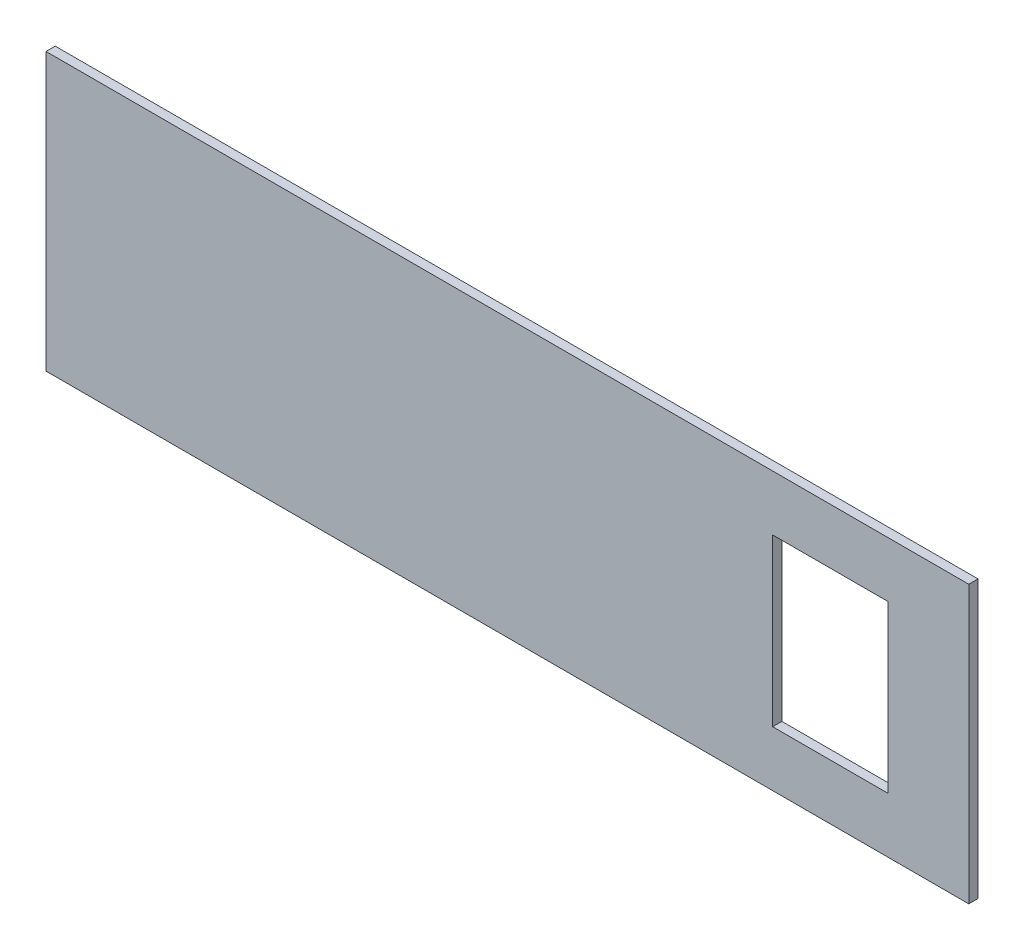
from build123d import *

# Parameters (mm, degrees)
SKETCH1_W              = 2000
SKETCH1_H              = 600
BOSS_EXTRUDE1_DEPTH    = 20
SKETCH2_W              = 250
SKETCH2_H              = 360
CUT_EXTRUDE1_DEPTH     = 1045.222198577
SKETCH3_W              = 60
SKETCH3_H              = 50
BOSS_EXTRUDE2_DEPTH    = 51
SKETCH4_W              = 60
SKETCH4_H              = 12
CUT_EXTRUDE2_DEPTH     = 40
FILLET1_R              = 12
SKETCH5_R              = 10
CUT_EXTRUDE3_DEPTH     = 1060.885489098
LPATTERN1_COUNT        = 2
LPATTERN1_PITCH        = 120
FILLET1_OF_LPATTERN1_R = 12


with BuildPart() as part:
    # Sketch1 → Boss-Extrude1 (new body)
    with BuildSketch(Plane.XY):
        Rectangle(SKETCH1_W, SKETCH1_H)
    extrude(amount=BOSS_EXTRUDE1_DEPTH)

    # Sketch2 → Cut-Extrude1 (cut, through all)
    with BuildSketch(Plane(origin=(0, 0, 0), x_dir=(-1, 0, 0), z_dir=(0, 0, -1))):
        with Locations((-700, 0)):
            Rectangle(SKETCH2_W, SKETCH2_H)
    extrude(amount=-CUT_EXTRUDE1_DEPTH, mode=Mode.SUBTRACT)

    # Sketch3 → Boss-Extrude2 (add)
    with BuildSketch(Plane(origin=(0, 0, 0), x_dir=(-1, 0, 0), z_dir=(0, 0, -1))):
        with Locations((-350, -22.5)):
            Rectangle(SKETCH3_W, SKETCH3_H)
    boss_extrude2 = extrude(amount=BOSS_EXTRUDE2_DEPTH)

    # Sketch4 → Cut-Extrude2 (cut)
    with BuildSketch(Plane(origin=(0, 0, -51), x_dir=(-1, 0, 0), z_dir=(0, 0, -1))):
        with Locations((-350, -23.5)):
            Rectangle(SKETCH4_W, SKETCH4_H)
    cut_extrude2 = extrude(amount=-CUT_EXTRUDE2_DEPTH, mode=Mode.SUBTRACT)

    # Fillet1
    fillet1_edges = [part.edges().sort_by_distance(p)[0] for p in [
        (380, -7.5, -51),
        (320, -38.5, -51),
        (380, -38.5, -51),
        (320, -7.5, -51),
    ]]
    fillet(fillet1_edges, radius=FILLET1_R)

    # Sketch5 → Cut-Extrude3 (cut, through all)
    with BuildSketch(Plane.XZ.offset(47.5)):
        with Locations((350, -26)):
            Circle(SKETCH5_R)
    cut_extrude3 = extrude(amount=-CUT_EXTRUDE3_DEPTH, mode=Mode.SUBTRACT)

    # LPattern1: Boss-Extrude2, Cut-Extrude2, Cut-Extrude3 ×2
    with Locations(*[(-i * LPATTERN1_PITCH, 0, 0) for i in range(1, LPATTERN1_COUNT)]):
        add(boss_extrude2)
        add(cut_extrude2, mode=Mode.SUBTRACT)
        add(cut_extrude3, mode=Mode.SUBTRACT)

    # Fillet1 of LPattern1
    fillet1_of_lpattern1_edges = [part.edges().sort_by_distance(p)[0] for p in [
        (260, -7.5, -51),
        (200, -38.5, -51),
        (260, -38.5, -51),
        (200, -7.5, -51),
    ]]
    fillet(fillet1_of_lpattern1_edges, radius=FILLET1_OF_LPATTERN1_R)


solid = part.part
